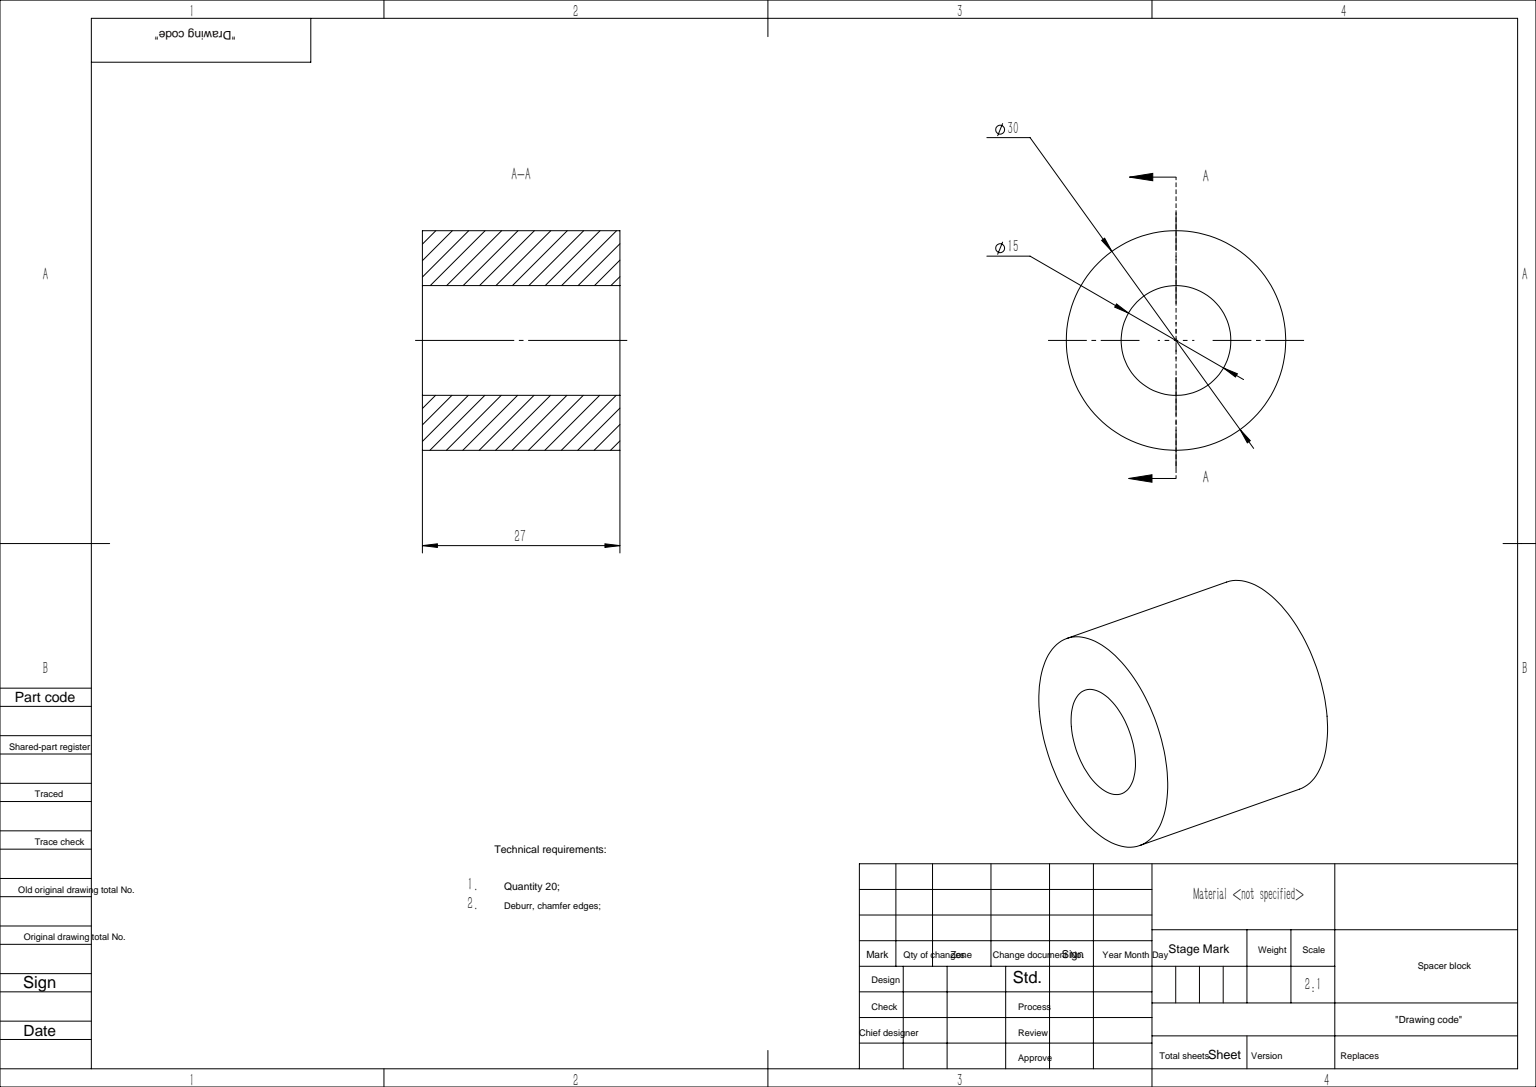
from build123d import *

# Parameters (mm, degrees)
SKETCH_1_R      = 15
SKETCH_1_R_2    = 7.5
EXTRUDE_1_DEPTH = 27


with BuildPart() as part:
    # 草图1 → 凸台-拉伸1 (new body)
    with BuildSketch(Plane(origin=(0, 0, -471), x_dir=(-1, 0, 0), z_dir=(0, 0, -1))):
        with Locations(Location((-645.939078063, 1570.019037425, 0), (0, 0, 180))):
            Circle(SKETCH_1_R)
        with Locations((-645.939078063, 1570.019037425)):
            Circle(SKETCH_1_R_2, mode=Mode.SUBTRACT)
    extrude(amount=EXTRUDE_1_DEPTH)


solid = part.part
